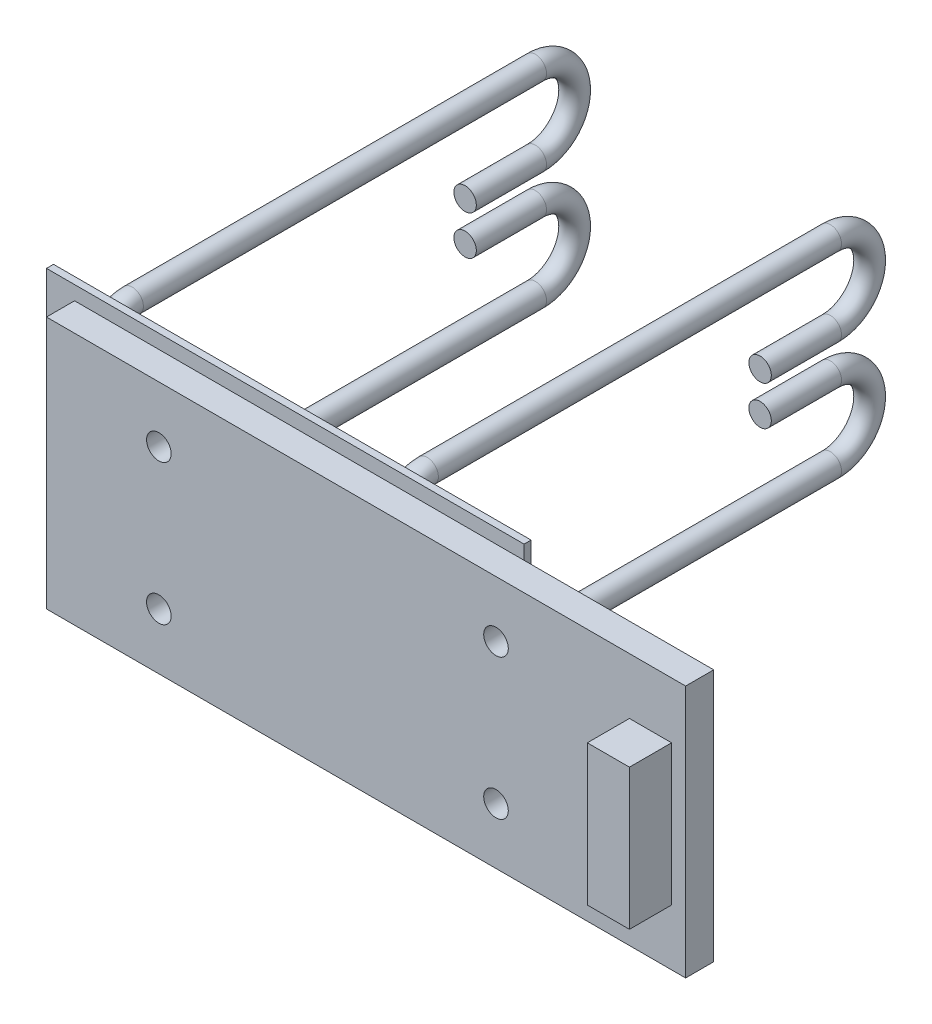
from build123d import *

# Parameters (mm, degrees)
SKETCH_1_W                   = 455
SKETCH_1_H                   = 180
EXTRUDE_1_DEPTH              = 20
SKETCH_2_W                   = 30
SKETCH_2_H                   = 100
EXTRUDE_2_DEPTH              = 30
SKETCH_3_W                   = 340
SKETCH_3_H                   = 200
EXTRUDE_3_DEPTH              = 5
SWEEP_1_PROFILE_R            = 8
PATTERN_LINEAR_1_COUNT       = 2
PATTERN_LINEAR_1_PITCH       = 210
HOLE_WIZARD_M20_1_AT_2_COUNT = 2
HOLE_WIZARD_M20_1_AT_2_PITCH = 240
HOLE_WIZARD_M20_1_AT_3_COUNT = 2
HOLE_WIZARD_M20_1_AT_3_PITCH = 260
HOLE_WIZARD_M20_1_AT_4_COUNT = 2
HOLE_WIZARD_M20_1_AT_4_PITCH = 100
SKETCH_8_W                   = 90
SKETCH_8_H                   = 140
EXTRUDE_4_DEPTH              = 3
PATTERN_LINEAR_2_COUNT       = 2
PATTERN_LINEAR_2_PITCH       = 240


with BuildPart() as part:
    # 草图1 → 凸台-拉伸1 (new body)
    with BuildSketch(Plane.XY):
        Rectangle(SKETCH_1_W, SKETCH_1_H)
    extrude(amount=EXTRUDE_1_DEPTH)


with BuildPart() as body_2:
    # 草图2 → 凸台-拉伸2 (new body)
    with BuildSketch(Plane.XY.offset(20)):
        with Locations((202.5, 0)):
            Rectangle(SKETCH_2_W, SKETCH_2_H)
    extrude(amount=EXTRUDE_2_DEPTH)


with BuildPart() as body_3:
    # 草图3 → 凸台-拉伸3 (new body)
    with BuildSketch(Plane(origin=(0, 0, 0), x_dir=(-1, 0, 0), z_dir=(0, 0, -1))):
        with Locations((77.5, 0)):
            Rectangle(SKETCH_3_W, SKETCH_3_H)
    extrude(amount=EXTRUDE_3_DEPTH)


with BuildPart() as body_4:
    # 扫描1: sweep along a path in 草图4
    with BuildLine(Plane.ZY.offset(227.5)) as sweep_1_path:
        Line((-278, 14), (-328, 14))
        ThreePointArc((-328, 14), (-356, 42), (-328, 70))
        Line((-328, 70), (-41, 70))
        ThreePointArc((-41, 70), (-21.201010127, 61.798989873), (-13, 42))
        Line((-13, 42), (-13, -42))
        ThreePointArc((-13, -42), (-21.201010127, -61.798989873), (-41, -70))
        Line((-41, -70), (-328, -70))
        ThreePointArc((-328, -70), (-356, -42), (-328, -14))
        Line((-328, -14), (-278, -14))
    # 扫描1 profile (on start of the path) → 扫描1 (sweep)
    with BuildSketch(Plane(origin=(-227.5, 14, -278), x_dir=(0, -1, 0), z_dir=(0, 0, -1))):
        Circle(SWEEP_1_PROFILE_R)
    sweep(path=sweep_1_path.line)


with BuildPart() as pattern_linear_1_1:
    # 阵列(线性)1: pattern copy
    add(body_4.part.moved(Location(Vector(1, 0, 0) * (1 * PATTERN_LINEAR_1_PITCH))))


with BuildPart() as hole_wizard_m20_1_tool:
    # 草图7 → M20 螺纹孔1 (revolve)
    with BuildSketch(Plane(origin=(92.5, -50, -5), x_dir=(0, 1, 0), z_dir=(1, 0, 0))):
        Polygon((0, 0), (0, 57.757530416), (8.75, 52.5), (8.75, 0), align=None)
    hole_wizard_m20_1 = revolve(axis=Axis((92.5, -50, -11.35), (0, 0, 1)))


with BuildPart() as part_1:
    add(part.part)

    # M20 螺纹孔1: cut by hole_wizard_m20_1_tool
    add(hole_wizard_m20_1_tool.part, mode=Mode.SUBTRACT)


with BuildPart() as body_3_1:
    add(body_3.part)

    # M20 螺纹孔1: cut by hole_wizard_m20_1_tool
    add(hole_wizard_m20_1_tool.part, mode=Mode.SUBTRACT)


with BuildPart() as hole_wizard_m20_1_at_2_tool:
    # M20 螺纹孔1 at 2: M20 螺纹孔1 ×2
    with Locations(*[(-i * HOLE_WIZARD_M20_1_AT_2_PITCH, 0, 0) for i in range(1, HOLE_WIZARD_M20_1_AT_2_COUNT)]):
        add(hole_wizard_m20_1)


with BuildPart() as part_2:
    add(part_1.part)

    # M20 螺纹孔1 at 2: cut by hole_wizard_m20_1_at_2_tool
    add(hole_wizard_m20_1_at_2_tool.part, mode=Mode.SUBTRACT)


with BuildPart() as body_3_2:
    add(body_3_1.part)

    # M20 螺纹孔1 at 2: cut by hole_wizard_m20_1_at_2_tool
    add(hole_wizard_m20_1_at_2_tool.part, mode=Mode.SUBTRACT)


with BuildPart() as hole_wizard_m20_1_at_3_tool:
    # M20 螺纹孔1 at 3: M20 螺纹孔1 ×2
    with Locations(*[Vector(-0.9230769230769229, 0.3846153846153851, 0) * (i * HOLE_WIZARD_M20_1_AT_3_PITCH) for i in range(1, HOLE_WIZARD_M20_1_AT_3_COUNT)]):
        add(hole_wizard_m20_1)


with BuildPart() as part_3:
    add(part_2.part)

    # M20 螺纹孔1 at 3: cut by hole_wizard_m20_1_at_3_tool
    add(hole_wizard_m20_1_at_3_tool.part, mode=Mode.SUBTRACT)


with BuildPart() as body_3_3:
    add(body_3_2.part)

    # M20 螺纹孔1 at 3: cut by hole_wizard_m20_1_at_3_tool
    add(hole_wizard_m20_1_at_3_tool.part, mode=Mode.SUBTRACT)


with BuildPart() as hole_wizard_m20_1_at_4_tool:
    # M20 螺纹孔1 at 4: M20 螺纹孔1 ×2
    with Locations(*[(0, i * HOLE_WIZARD_M20_1_AT_4_PITCH, 0) for i in range(1, HOLE_WIZARD_M20_1_AT_4_COUNT)]):
        add(hole_wizard_m20_1)


with BuildPart() as part_4:
    add(part_3.part)

    # M20 螺纹孔1 at 4: cut by hole_wizard_m20_1_at_4_tool
    add(hole_wizard_m20_1_at_4_tool.part, mode=Mode.SUBTRACT)


with BuildPart() as body_3_4:
    add(body_3_3.part)

    # M20 螺纹孔1 at 4: cut by hole_wizard_m20_1_at_4_tool
    add(hole_wizard_m20_1_at_4_tool.part, mode=Mode.SUBTRACT)


with BuildPart() as body_6:
    # 草图8 → 凸台-拉伸4 (new body)
    with BuildSketch(Plane(origin=(0, 0, -5), x_dir=(-1, 0, 0), z_dir=(0, 0, -1))):
        with Locations((162.5, 0)):
            Rectangle(SKETCH_8_W, SKETCH_8_H)
    extrude(amount=EXTRUDE_4_DEPTH)


with BuildPart() as pattern_linear_2_1:
    # 阵列(线性)2: pattern copy
    add(body_6.part.moved(Location(Vector(1, 0, 0) * (1 * PATTERN_LINEAR_2_PITCH))))


solid = Compound([body_2.part, body_4.part, pattern_linear_1_1.part, part_4.part, body_3_4.part, body_6.part, pattern_linear_2_1.part])
